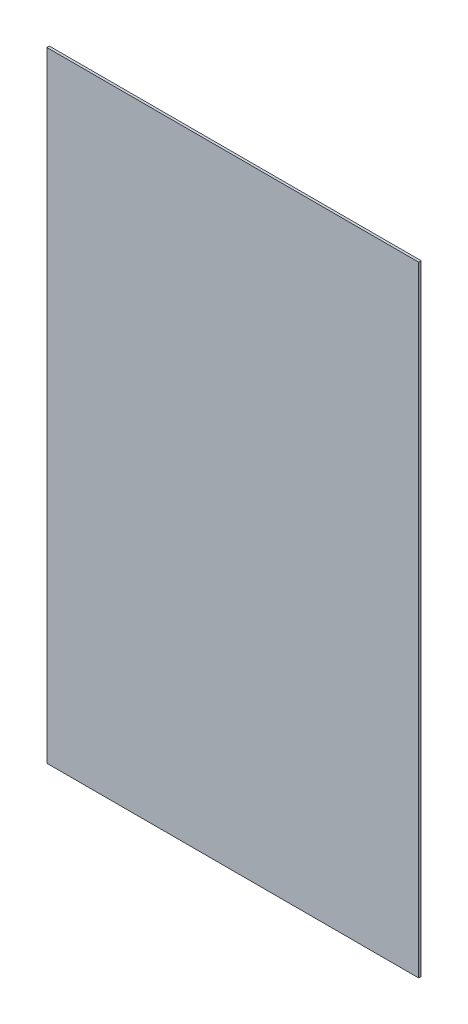
from build123d import *

# Parameters (mm, degrees)
SKETCH_1_W      = 30
SKETCH_1_H      = 50
EXTRUDE_1_DEPTH = 0.2


with BuildPart() as part:
    # 草图1 → 凸台-拉伸1 (new body)
    with BuildSketch(Plane.XY):
        Rectangle(SKETCH_1_W, SKETCH_1_H)
    extrude(amount=EXTRUDE_1_DEPTH)


solid = part.part
